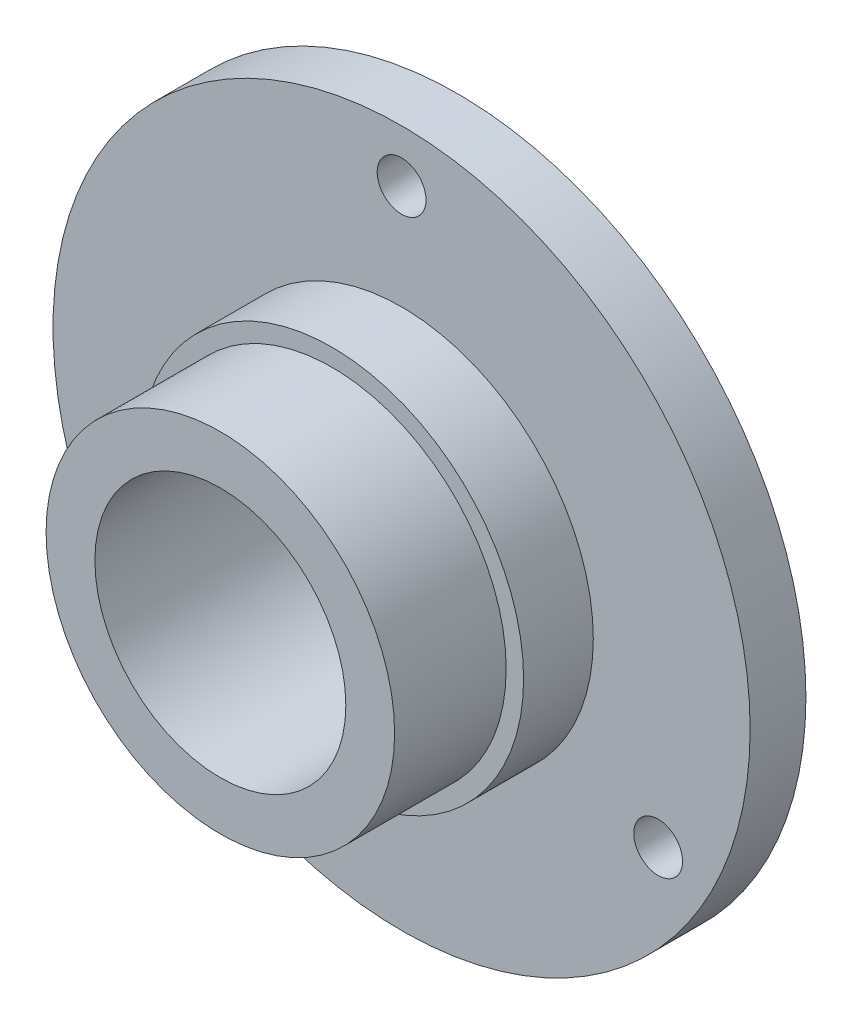
from build123d import *

# Parameters (mm, degrees)
SKETCH1_R           = 50
SKETCH1_R_2         = 3.5
SKETCH1_R_3         = 18
BOSS_EXTRUDE1_DEPTH = 8
SKETCH2_R           = 27.5
SKETCH2_R_2         = 18
BOSS_EXTRUDE2_DEPTH = 10
SKETCH3_R           = 25
SKETCH3_R_2         = 18
BOSS_EXTRUDE3_DEPTH = 16


with BuildPart() as part:
    # Sketch1 → Boss-Extrude1 (new body)
    with BuildSketch(Plane.XY):
        Circle(SKETCH1_R)
        with Locations((0, 42.5)):
            Circle(SKETCH1_R_2, mode=Mode.SUBTRACT)
        with Locations((-36.806079661, -21.25)):
            Circle(SKETCH1_R_2, mode=Mode.SUBTRACT)
        with Locations((36.806079661, -21.25)):
            Circle(SKETCH1_R_2, mode=Mode.SUBTRACT)
        Circle(SKETCH1_R_3, mode=Mode.SUBTRACT)
    extrude(amount=BOSS_EXTRUDE1_DEPTH)

    # Sketch2 → Boss-Extrude2 (add)
    with BuildSketch(Plane.XY.offset(8)):
        Circle(SKETCH2_R)
        Circle(SKETCH2_R_2, mode=Mode.SUBTRACT)
    extrude(amount=BOSS_EXTRUDE2_DEPTH)

    # Sketch3 → Boss-Extrude3 (add)
    with BuildSketch(Plane.XY.offset(18)):
        Circle(SKETCH3_R)
        Circle(SKETCH3_R_2, mode=Mode.SUBTRACT)
    extrude(amount=BOSS_EXTRUDE3_DEPTH)


solid = part.part
